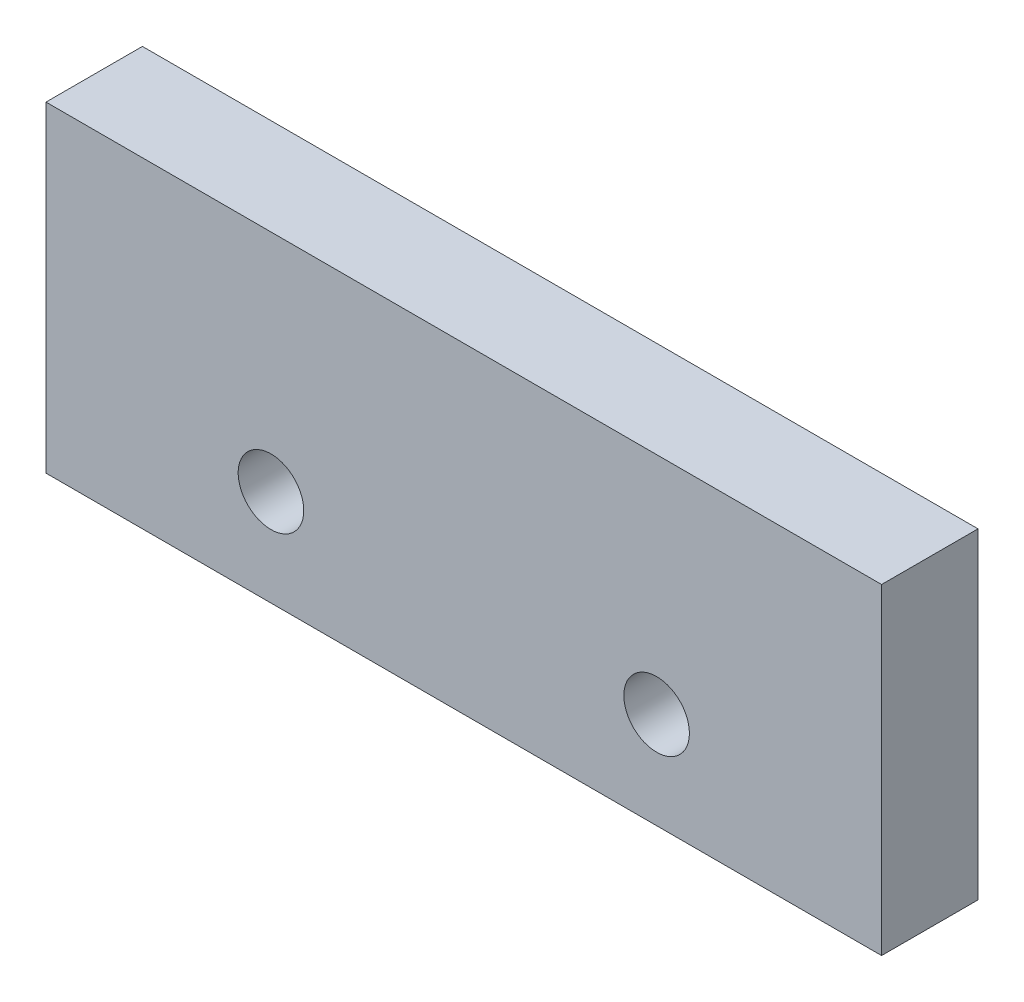
SolidWorks part; units mm, degrees
material "1023 碳钢板 (SS)"
ref_plane "Front Plane" through (0, 0, 0) normal (0, 0, 1) x (1, 0, 0)
ref_plane "Top Plane" through (0, 0, 0) normal (0, 1, 0) x (1, 0, 0)
ref_plane "Right Plane" through (0, 0, 0) normal (1, 0, 0) x (0, 0, -1)
sketch "Sketch1" plane through (0, 0, 0) normal (0, 0, 1) x (1, 0, 0)
  line L1 (-65, 25) -> (65, 25)
  line L2 (-65, 25) -> (-65, -25)
  line L3 (-65, -25) -> (65, -25)
  line L4 (65, 25) -> (65, -25)
  line L5 (-65, 25) -> (65, -25) construction
  line L6 (-65, -25) -> (65, 25) construction
  point P0 (0, 0)
  dimension "D1" = 130
  dimension "D2" = 50
extrude "Boss-Extrude1" add sketch "Sketch1" along normal blind 15
sketch "Sketch2" plane through (0, 0, 15) normal (0, 0, 1) x (1, 0, 0)
  line L0 (-65, -25) -> (65, -25) construction
  line L1 (65, -25) -> (65, 25) construction
  circle A2 centre (-30, -10) radius 16.1483
  circle A3 centre (30, -10) radius 7.112
  dimension "D1" = 60
  dimension "D3" = 15
  dimension "D2" = 35
hole_wizard "M12 Tapped Hole1" positions "Sketch3" profile "Sketch4" tap size "M12" standard "ISO"
sketch "Sketch3" plane through (0, 0, 15) normal (0, 0, 1) x (1, 0, 0)
  point P0 (-30, -10)
  point P3 (30, -10)
sketch "Sketch4" plane through (-30, -10, 15) normal (1, 0, 0) x (0, -1, 0)
  line L0 (0, 0) -> (0, 32.3144)
  line L1 (0, 32.3144) -> (5.1, 29.25)
  line L2 (5.1, 29.25) -> (5.1, 0)
  line L5 (5.1, 0) -> (0, 0)
  line L10 (0, 32.3144) -> (-5.1, 29.25) construction
  line L11 (0, -6.35) -> (0, 107.95) construction
  dimension "螺纹孔钻头直径" = 10.2
  dimension "螺纹孔钻头深度" = 29.25
  dimension "导头角度" = 118
cosmetic thread "Hole Thread Line1" parameters "D1"=24, "D2"=12
cosmetic thread "Hole Thread Line2" parameters "D1"=24, "D2"=12
